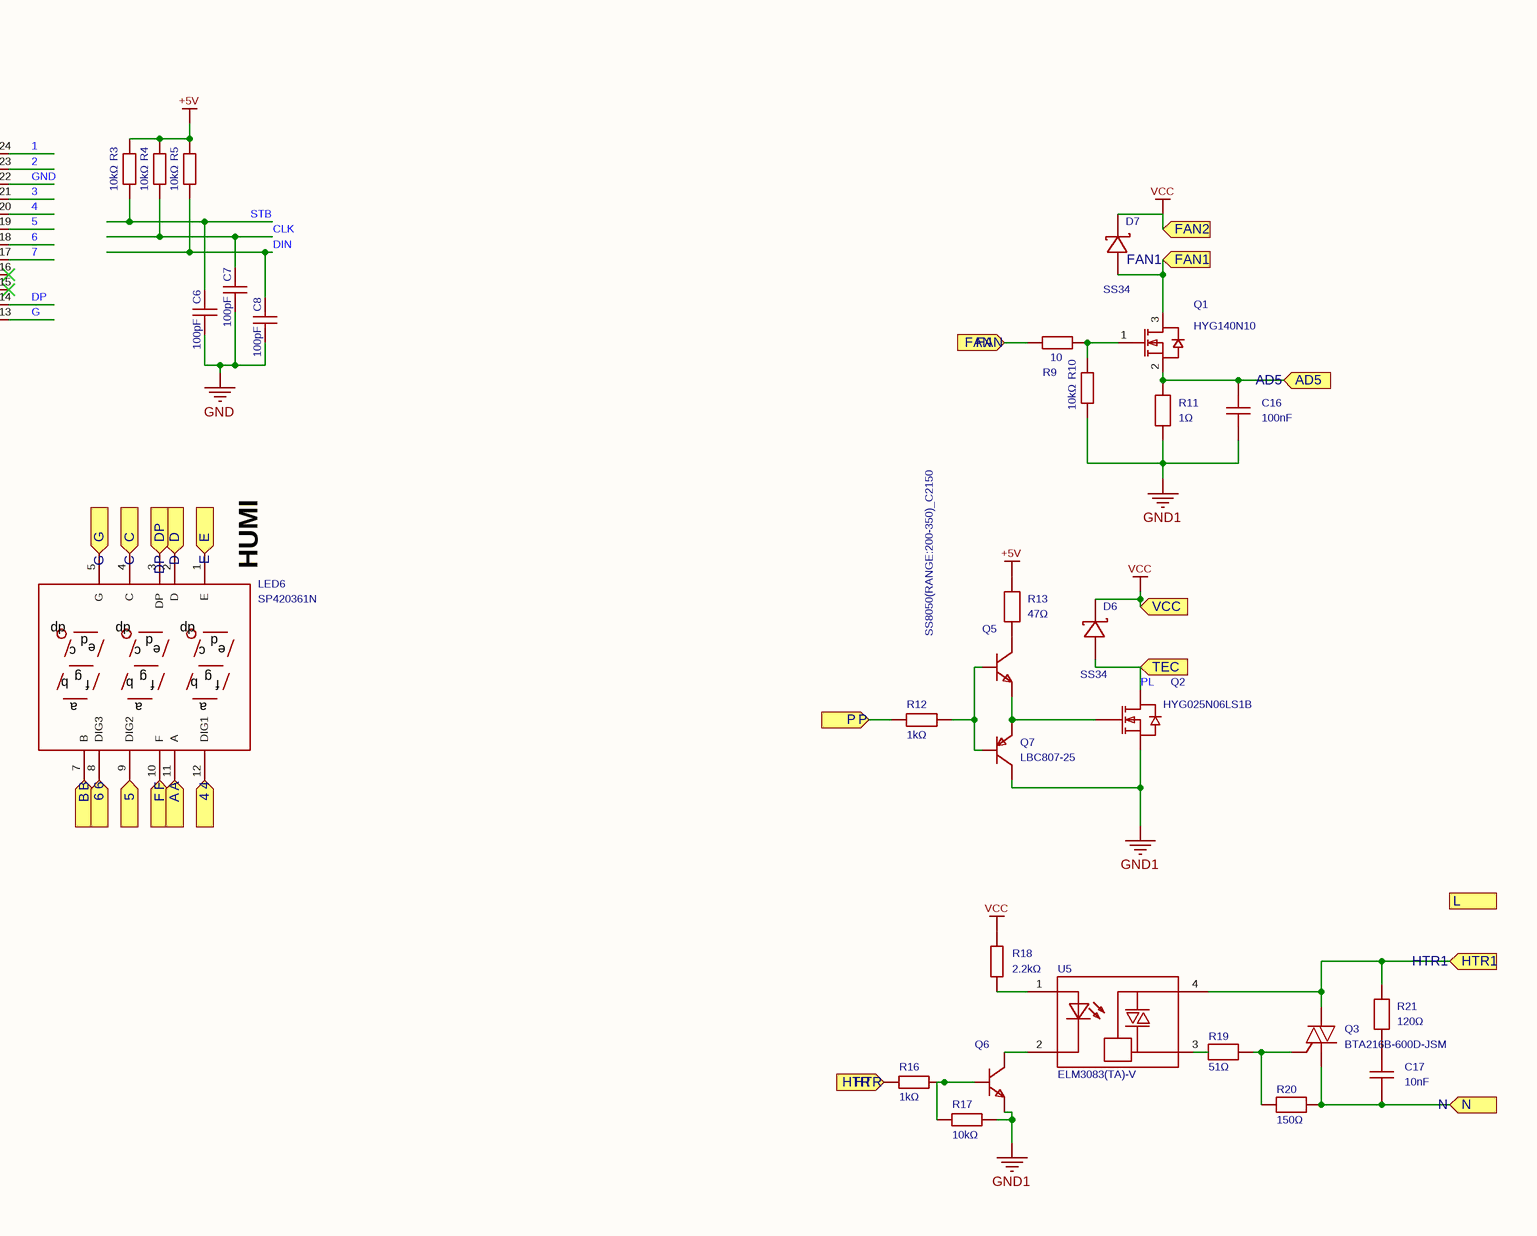
[diagram p0: MISC84275-2.SchDoc, right]
# Altium project MISC84275.PrjPcb (part 2 of 2)
## Sheet MISC84275-2.SchDoc (continued)
### Library data of the parts (continued)
D2 = SS34_C8678: Diode configuration:Single;Forward voltage(Vf):550mV@3A;DC reverse voltage(Vr):40V;Rectified current:3A;; Manufacturer: MDD(辰达半导体); AddInBom: yes; ModelId: e3551acb3c5a4975a5e9d36087fe1fa2; ModelTransform: 185.039,102.362,0,0,0,0,0,0,0; Diode Configuration: Single; Voltage - DC Reverse(Vr): 40V; Current - Rectified: 3A; Reverse Leakage Current (Ir): 500uA@40V; Operating Junction Temperature Range: -55℃~+125℃; Symbol: SS34_C8678; Device: SS34_C8678; LCSC Part Name: 电压:40V 电流:3A; SupplierPart: C8678; ManufacturerPart: SS34; Supplier Footprint: SMA(DO-214AC); JLCPCB Part Class: Basic library; Datasheet: https://item.szlcsc.com/datasheet/SS34/9178.html; Supplier: LCSC; ConvertToPcb: yes; FootprintName: SMA_L4.3-W2.6-LS5.2-RD; ModelName: SMA_L4.3-W2.6-LS5.2-RD; Voltage - Forward(Vf@If): 550mV@3A
D3-D5 = SMF36CA_C435502: Polarity:Bidirectional;Reverse standoff voltage(Vrwm):36V;Clamping voltage:58.1V;Peak pulse current(Ipp):3.5A;Peak pulse power(Ppp):200W@10/1000us;Breakdown voltage:40V;; Manufacturer: AnBon(安邦); 3D Model: 8576f175c34f41329e79954aa68cc529; 3D Model Transform: 145.669,70.866,0,0,0,0,0,0,0; Reverse Stand-Off Voltage (Vrwm): 36V; Clamping Voltage: 58.1V; Peak Pulse Current (Ipp): 3.5A; Voltage - Breakdown: 40V; Reverse Leakage Current (Ir): 5uA; Number of Channels: Single channel; Type: TVS; AddInBom: yes; Symbol: SMF36CA_C435502; Device: SMF36CA_C435502; LCSC Part Name: SMF36CA; Supplier Part: C435502; Manufacturer Part: SMF36CA; Supplier Footprint: SOD-123; JLCPCB Part Class: Extended library; Datasheet: https://item.szlcsc.com/datasheet/SMF36CA/432840.html; Supplier: LCSC; Polarity: Bidirectional; Peak Pulse Power Dissipation (Ppp): 200W@10/1000us; Operating Temperature: -55℃~+150℃; ConvertToPcb: yes; FootprintName: SOD-123_L2.7-W1.8-LS3.7-BI; ModelName: SOD-123_L2.7-W1.8-LS3.7-BI
D6 D7 = SS34_C8678: Diode configuration:Single;Forward voltage(Vf):550mV@3A;DC reverse voltage(Vr):40V;Rectified current:3A;; Manufacturer: MDD(辰达半导体); 3D Model: e3551acb3c5a4975a5e9d36087fe1fa2; 3D Model Transform: 185.039,102.362,0,0,0,0,0,0,0; Diode Configuration: Single; Voltage - DC Reverse(Vr): 40V; Current - Rectified: 3A; Reverse Leakage Current (Ir): 500uA@40V; Operating Junction Temperature Range: -55℃~+125℃; AddInBom: yes; Symbol: SS34_C8678; Device: SS34_C8678; LCSC Part Name: 电压:40V 电流:3A; Supplier Part: C8678; Manufacturer Part: SS34; Supplier Footprint: SMA(DO-214AC); JLCPCB Part Class: Basic library; Datasheet: https://item.szlcsc.com/datasheet/SS34/9178.html; Supplier: LCSC; Voltage - Forward(Vf@If): 550mV@3A; ConvertToPcb: yes; FootprintName: SMA_L4.3-W2.6-LS5.2-RD; ModelName: SMA_L4.3-W2.6-LS5.2-RD
FAN FAN2 = XH2.54-2P立贴: AddInBom: yes; ModelId: fc9104ee8bac4316b59c074360305c900819f05c4eef4c71ace90d822a990e87; ModelTransform: 393.7,326.771,0,0,0,0,0,9.966,0; Symbol: XH2.54-2P vertical SMD; Device: XH2.54-2P vertical SMD; LCSC Part Name: XH2.54-2P立贴; SupplierPart: C9900007402; ManufacturerPart: XH2.54-2P立贴; Supplier Footprint: XH2.5-2P母座立贴; JLCPCB Part Class: Extended Part; Supplier: LCSC; ConvertToPcb: yes; FootprintName: CONN-SMD_2P_A2501WV-S; ModelName: CONN-SMD_2P_A2501WV-S
H1 = PZ254V-11-04P: Pin structure:1x4P;Pitch:2.54mm;Row spacing:-;Round/square pin:Square pin;Mounting:Through-hole;Rows:Single row;Total pins:4P;Rated current:3A;Rated voltage:250V;Mating pin length:6mm;Body height:2.5mm;Tail length:3mm;Contact material:-;Operating temp:-40℃~+105℃;Colour:Black;; Manufacturer: XFCN(兴飞); Symbol: PZ254V-11-04P_C2691448; AddInBom: yes; ModelId: 112f4d05e8d64e99ab9a333894bea4f9; ModelName: HDR-TH_4P-P2.54-M-LI-1X4P; ModelTransform: 399.999,104.7242,0,0,0,0,0,0,-118.11; Pin Structure: 1x4P; Pitch: 2.54mm; Current Rating: 3A; Voltage Rating (Max): 250V; Device: PZ254V-11-04P; LCSC Part Name: 1x4P 间距:2.54mm 方针 直插; SupplierPart: C2691448; ManufacturerPart: PZ254V-11-04P; Supplier Footprint: 插件,P=2.54mm; JLCPCB Part Class: Extended library; Datasheet: https://item.szlcsc.com/datasheet/PZ254V-11-04P/2801085.html; Supplier: LCSC; ConvertToPcb: yes; FootprintName: HDR-TH_4P-P2.54-V-M; Row Spacing: -; Circluar Pins/Square Pins: Square pin; Mounting Type: Through-hole; Number of Rows: Single row; Number of Pins: 4P; Length of Mating Pin: 6mm; Insulation Height: 2.5mm; Length of End Connection Pin: 3mm; Contact Material: -; Operating Temperature: -40℃~+105℃; Color: Black
HTR = VH3.96-3P: AddInBom: yes; ModelId: 84617fe1842943989a766f28ebeae3030819f05c4eef4c71ace90d822a990e87; ModelTransform: 623.6208,484.251,0,0,0,0,0.001,0.984,0; Symbol: VH3.96-3P; Device: VH3.96-3P; LCSC Part Name: VH3.96-3P; SupplierPart: C9900014650; ManufacturerPart: VH3.96-3P; Supplier Footprint: VH3.963P贴; JLCPCB Part Class: Extended Part; Supplier: LCSC; ConvertToPcb: yes; FootprintName: CONN-SMD_3P-P3.96_HCTL_HC-VH-3ALT; ModelName: CONN-SMD_3P-P3.96_HCTL_HC-VH-3ALT
L1 = PSPMAA0605H-680M-IGF: Inductance:68uH;Tolerance:±20%;Rated current:1.5A;Saturation current(Isat):2A;Type:-;; Manufacturer: PROD(谱罗德); 3D Model: 42305e89796f47b49312a685ea93d4940819f05c4eef4c71ace90d822a990e87; 3D Model Transform: 275.59,259.88137,0,0,0,0,0,-0.551,0; Tolerance: ±20%; Current Rating: 1.5A; Current - Saturation(Isat): 2A; DC Resistance(DCR): 256mΩ; AddInBom: yes; ModelName: IND-SMD_L7.1-W6.6-H5.0; Symbol: PSPMAA0605H-680M-IGF; Device: PSPMAA0605H-680M-IGF; LCSC Part Name: 68uH ±20% 2A; Supplier Part: C2983094; Manufacturer Part: PSPMAA0605H-680M-IGF; Supplier Footprint: SMD,7.1x6.6mm; JLCPCB Part Class: Extended Part; Datasheet: https://item.szlcsc.com/datasheet/PSPMAA0605H-680M-IGF/3416346.html; Supplier: LCSC; Value: 68uH; Type: -; Ratings: -; ConvertToPcb: yes; FootprintName: IND-SMD_L7.1-W6.6_H5.0
L2 L3 = SCL3216T220KSP: Inductance:22uH;Tolerance:±10%;Rated current:5mA;Saturation current(Isat):-;DC resistance(DCR):900mΩ;; Manufacturer: Sunltech(顺磁); 3D Model: 85bdab7b3d4c4074b81d208eb5e865b30819f05c4eef4c71ace90d822a990e87; 3D Model Transform: 125.984,62.835,0,0,0,0,0,0,0; Tolerance: ±10%; Current Rating: 5mA; DC Resistance(DCR): 900mΩ; AddInBom: yes; ModelName: L1206_L3.2-W1.6-H1.1; Symbol: SCL3216T220KSP; Device: SCL3216T220KSP; LCSC Part Name: 22uH ±10%; Supplier Part: C412019; Manufacturer Part: SCL3216T220KSP; Supplier Footprint: 1206; JLCPCB Part Class: Extended Part; Datasheet: https://item.szlcsc.com/datasheet/SCL3216T220KSP/403512.html; Supplier: LCSC; Value: 22uH; Current - Saturation (Isat): -; Q @ Frequency: -; Frequency - Self Resonant: -; Ratings: -; ConvertToPcb: yes; FootprintName: L1206
LED1-LED4 = 3mmFIR: 3D Model: a497c992633541038a38947cdc58012f; 3D Model Transform: 141.274,153.327,0,0,0,0,-5.984,0,-137.795; AddInBom: yes; ModelName: LED-TH-3mm_R; Symbol: 3MMFIR; Device: 3mmFIR; LCSC Part Name: 3mmFIR; Supplier Part: C9900095018; Manufacturer Part: 3mmFIR; Supplier Footprint: LED-TH_LED-3MM_RED; JLCPCB Part Class: Extended library; Supplier: LCSC; ConvertToPcb: yes; FootprintName: LED-TH_BD3.0-P2.54-FD
LED5 LED6 = EPHB_SP420361N 0.36英寸3位红色数码管: Same display size as the 30V tester I bought, Digits:3 digits;Emitting colour:Red;LED polarity:Common cathode;Character height (inch):0.36;; Manufacturer: ARKLED(方舟); Device: EPHB_SP420361N 0.36 inch 3 digit red seven-segment display; 3D Model: 75b7188ef1934ceeb211c7922abf127e; 3D Model Transform: 885.825,551.5737,0,90,0,0,0,0,-196.85; Luminous Color: Red; Digit/Alpha Size(inch): 0.36; AddInBom: yes; Symbol: SP420361N; Manufacturer Part: SP420361N; Supplier: LCSC; Supplier Part: C98927; LCSC Part Name: 3位0.36英寸红色数码管 共阴极; Supplier Footprint: 插件; JLCPCB Part Class: Extended Part; Datasheet: https://atta.szlcsc.com/upload/public/pdf/source/20170713/C98927_1499918920582816853.pdf; Number of Characters: 3 digits; LED Polarity: Common cathode; ConvertToPcb: yes; FootprintName: LED-SEG-TH_SP420361N; ModelName: LED-SEG-TH_SP420361N
Q1 = NCE0140K2-VB: Type:1 N-channel;Drain-source voltage(Vdss):100V;Continuous drain current(Id):45A;On-resistance(RDS(on)@Vgs,Id):-;Power(Pd):3W;Threshold voltage(Vgs(th)@Id):2.5V@250uA;; Manufacturer: VBsemi(微碧半导体); 3D Model: 002f14490d3e47dc80a93c97f5a1e7bb; 3D Model Transform: 385.5088,255.905,0,0,0,0,-33.661,0,0; Drain Source Voltage (Vdss): 100V; Continuous Drain Current (Id): 45A; Power Dissipation (Pd): 3W; Total Gate Charge (Qg@Vgs): 38nC@10V; Input Capacitance (Ciss@Vds): 2.4nF@50V; Reverse Transfer Capacitance (Crss@Vds): 80pF@50V; AddInBom: yes; Symbol: NCE0140K2-VB; Device: NCE0140K2-VB; Manufacturer Part: HYG140N10; LCSC Part Name: 1个N沟道 耐压:100V 电流:45A; Supplier Part: C7463473; Supplier Footprint: TO-252; JLCPCB Part Class: Extended library; Datasheet: https://atta.szlcsc.com/upload/public/pdf/source/20240821/DCE0DDCDA6E2F6C426FEF52E9193F584.pdf; Supplier: LCSC; Type: 1 N-channel; Drain Source On Resistance (RDS(on)@Vgs,Id): -; Gate Threshold Voltage (Vgs(th)@Id): 2.5V@250uA; Operating Temperature: -55℃~+175℃; ConvertToPcb: yes; FootprintName: TO-252-3_L6.6-W6.1-P4.58-LS10.1-BR; ModelName: TO-252-3_L6.6-W6.1-P4.58-LS10.1-BR
Q2 = HYG025N06LS1B: Quantity:1 N-channel;Drain-source voltage(Vdss):60V;Continuous drain current(Id):160A;On-resistance(RDS(on)):3.3mΩ@10V;Power dissipation(Pd):125W;Threshold voltage(Vgs(th)):3V@250uA;; Manufacturer: HUAYI(华羿微); 3D Model: e74d9d1f92e14ef38b829eb45550a5f50819f05c4eef4c71ace90d822a990e87; 3D Model Transform: 399.999,594.487,0,90,0,0,-25.236,0,0; Drain to Source Voltage: 60V; Current - Continuous Drain(Id): 160A; Pd - Power Dissipation: 125W; Gate Charge(Qg): 58.3nC@10V; Input Capacitance(Ciss): 3.915nF; Reverse Transfer Capacitance (Crss@Vds): 10.2pF; Output Capacitance(Coss): 1.31nF; AddInBom: yes; Symbol: HYG025N06LS1B; Device: HYG025N06LS1B; LCSC Part Name: 1个N沟道 耐压:60V 电流:160A; Supplier Part: C2836680; Manufacturer Part: HYG025N06LS1B; Supplier Footprint: TO-263-2L; JLCPCB Part Class: Extended Part; Datasheet: https://item.szlcsc.com/datasheet/HYG025N06LS1B/3004274.html; Supplier: LCSC; Number: 1 N-channel; RDS(on): 3.3mΩ@10V; Gate Threshold Voltage (Vgs(th)): 3V@250uA; Operating Temperature: -55℃~+175℃; Type: N-channel; ConvertToPcb: yes; FootprintName: TO-263-2_L10.2-W8.7-P5.08-LS15.1-BR; ModelName: TO-263-2_L10.2-W8.7-P5.08-LS15.1-BR
Q3 = BTA216B-600D-JSM: Holding current(Ih):25mA;Off-state peak voltage(Vdrm):600V;Gate trigger current(Igt):50mA;; Manufacturer: JSMSEMI(杰盛微); 3D Model: 74c353bcc44b4c868478fa9e8b3e61680819f05c4eef4c71ace90d822a990e87; 3D Model Transform: 393.7,606.298,0,90,0,0,-49.213,0,0; Gate Trigger   Voltage (Vgt): 1.3V; Holding Current (Ih): 25mA; Peak off - state voltage(Vdrm): 600V; Current - Gate Trigger(Igt): 50mA; Voltage - On State(Vtm): 1.55V; Current - On State(It(RMS)): 16A; AddInBom: yes; Symbol: BTA216B-600D-JSM; Device: BTA216B-600D-JSM; LCSC Part Name: 16A无缓冲器三端双向可控硅; Supplier Part: C18189168; Manufacturer Part: BTA216B-600D-JSM; Supplier Footprint: TO-263; JLCPCB Part Class: Extended Part; Datasheet: https://item.szlcsc.com/datasheet/BTA216B-600D-JSM/19338246.html; Supplier: LCSC; ConvertToPcb: yes; FootprintName: TO-263-3_L10.2-W9.2-P5.08-LS15.4-BR; ModelName: TO-263-3_L10.2-W9.2-P5.08-LS15.4-BR
Q4-Q6 = SS8050(RANGE:200-350)_C2150: Transistor type:NPN;Collector current(Ic):1.5A;C-E breakdown voltage(Vceo):25V;Power(Pd):300mW;DC current gain(hFE@Ic,Vce):200@800mA,1V;; Manufacturer: CJ(江苏长电/长晶); Symbol: SS8050_C2150; 3D Model: c62791f0466c4ae2a892c056b845b0ca; 3D Model Transform: 98.425,114.173,0,180,0,0,0.0005,-0.0005,0; Transistor Type: NPN; Collector Current (Ic): 1.5A; Collector-Emitter Breakdown Voltage (Vceo): 25V; Power Dissipation (Pd): 300mW; Transition Frequency (fT): 100MHz; Collector Cut-Off Current (Icbo): 100nA; Collector-Emitter Saturation Voltage (VCE(sat)@Ic,Ib): 500mV@800mA,80mA; AddInBom: yes; ModelName: SOT-23-3P_L2.9-W1.3-H1.0-LS2.4-P0.95; Device: SS8050(RANGE:200-350)_C2150; LCSC Part Name: NPN 电流:1.5A 耐压:25V hfe=200~350; Supplier Part: C2150; Manufacturer Part: SS8050(RANGE:200-350); Supplier Footprint: SOT-23; JLCPCB Part Class: Basic library; Datasheet: https://atta.szlcsc.com/upload/public/pdf/source/20230322/AEE86F4B043774EFF80CAEA14A37D9E9.pdf; Supplier: LCSC; DC Current Gain (hFE@Ic,Vce): 200@800mA,1V; Operating Temperature: -55℃~+150℃; ConvertToPcb: yes; FootprintName: SOT-23-3_L2.9-W1.3-P1.90-LS2.4-BR
Q7 = LBC807-25LT1G: Transistor type:PNP;Collector current(Ic):500mA;C-E breakdown voltage(Vceo):45V;Power(Pd):225mW;DC current gain(hFE@Ic,Vce):160@100mA,1.0V;; Manufacturer: LRC(乐山无线电); 3D Model: 89cb27a44ab2466697082bb9fd73a7d0; 3D Model Transform: 114.173,110.236,0,90,0,0,0,0,0; Transistor Type: PNP; Collector Current (Ic): 500mA; Collector-Emitter Breakdown Voltage (Vceo): 45V; Power Dissipation (Pd): 225mW; Transition Frequency (fT): 100MHz; Collector Cut-Off Current (Icbo): 5uA; Collector-Emitter Saturation Voltage (VCE(sat)@Ic,Ib): 700mV@500mA,50mA; AddInBom: yes; ModelName: SOT-23-3L_L2.9-W1.6-H1.1-LS2.8-P0.95; Symbol: LBC807-25LT1G; Device: LBC807-25LT1G; Manufacturer Part: LBC807-25; LCSC Part Name: PNP 电流:500mA 耐压:45V hfe=160~400; Supplier Part: C12781; Supplier Footprint: SOT-23; JLCPCB Part Class: Extended library; Datasheet: https://atta.szlcsc.com/upload/public/pdf/source/20190627/C383184_22DCACC56563C88F03CAC9F09322D9FA.pdf; Supplier: LCSC; DC Current Gain (hFE@Ic,Vce): 160@100mA,1.0V; Operating Temperature: -55℃~+150℃; ConvertToPcb: yes; FootprintName: SOT-23-3_L2.9-W1.6-P1.90-LS2.8-BR
R1 R2 R12 R16 R23 = 0805W8F1001T5E: Resistor type:Thick film resistor;Resistance:1kΩ;Tolerance:±1%;Power:125mW;Max operating voltage:150V;Temp coefficient:±100ppm/℃;; Manufacturer: UNI-ROYAL(厚声); 3D Model: 37a81e68749a4138bd2dfa6897b24b850819f05c4eef4c71ace90d822a990e87; 3D Model Transform: 78.74,51.181,0,0,0,0,0,-0.0005,0; Tolerance: ±1%; Power(Watts): 125mW; Overload Voltage (Max): 150V; AddInBom: yes; ModelName: R0805_L2.0-W1.3-H0.6; Symbol: 0805W8F1001T5E; Device: 0805W8F1001T5E; LCSC Part Name: 1kΩ ±1% 125mW 厚膜电阻; Manufacturer Part: 0805W8F1001T5E; Supplier Footprint: 0805; JLCPCB Part Class: Basic Part; Datasheet: https://atta.szlcsc.com/upload/public/pdf/source/20200306/C422600_1E6D84923E4A46A82E41ADD87F860B5C.pdf; Supplier: LCSC; Type: Thick film resistor; Temperature Coefficient: ±100ppm/℃; Operating Temperature Range: -55℃~+155℃; ConvertToPcb: yes; FootprintName: R0805
  R1: Value: 1K
  R2: Value: 10kΩ
  R12 R16 R23: Supplier Part: C17513; Value: 1kΩ
R3-R5 R10 R17 R22 = 0805W8F1002T5E_C17414: Resistor type:Thick film resistor;Resistance:10kΩ;Tolerance:±1%;Power:125mW;Operating voltage:150V;Temp coefficient:±100ppm/℃;; Manufacturer: UNI-ROYAL(厚声); 3D Model: 37a81e68749a4138bd2dfa6897b24b850819f05c4eef4c71ace90d822a990e87; 3D Model Transform: 78.74,51.181,0,0,0,0,0,-0.0005,0; Tolerance: ±1%; Power(Watts): 125mW; Voltage-Supply(Max): 150V; AddInBom: yes; ModelName: R0805_L2.0-W1.3-H0.6; Symbol: 0805W8F1002T5E; Device: 0805W8F1002T5E_C17414; LCSC Part Name: 10kΩ ±1% 125mW 厚膜电阻; Supplier Part: C17414; Manufacturer Part: 0805W8F1002T5E; Supplier Footprint: 0805; JLCPCB Part Class: Basic Part; Datasheet: https://item.szlcsc.com/datasheet/0805W8F1002T5E/18102.html; Supplier: LCSC; Type: Thick film resistor; Value: 10kΩ; Temperature Coefficient: ±100ppm/℃; Operating Temperature: -55℃~+155℃; ConvertToPcb: yes; FootprintName: R0805
R6 R8 = 0805W8F4702T5E: Resistor type:Thick film resistor;Resistance:47kΩ;Tolerance:±1%;Power:125mW;Max operating voltage:150V;Temp coefficient:±100ppm/℃;; Manufacturer: UNI-ROYAL(厚声); 3D Model: 37a81e68749a4138bd2dfa6897b24b85; 3D Model Transform: 78.74,51.181,0,0,0,0,0,-0.0005,0; Tolerance: ±1%; Power(Watts): 125mW; Overload Voltage (Max): 150V; AddInBom: yes; ModelName: R0805_L2.0-W1.3-H0.6; Symbol: 0805W8F4702T5E; Device: 0805W8F4702T5E; LCSC Part Name: 47kΩ ±1% 125mW 厚膜电阻; Supplier Part: C17713; Manufacturer Part: 0805W8F4702T5E; Supplier Footprint: 0805; JLCPCB Part Class: Basic Part; Datasheet: https://atta.szlcsc.com/upload/public/pdf/source/20200306/C422600_1E6D84923E4A46A82E41ADD87F860B5C.pdf; Supplier: LCSC; Type: Thick film resistor; Value: 47kΩ; Temperature Coefficient: ±100ppm/℃; Operating Temperature Range: -55℃~+155℃; ConvertToPcb: yes; FootprintName: R0805
R7 = FRC0805F1202TS: Resistor type:Thick film resistor;Resistance:12kΩ;Tolerance:±1%;Power:125mW;Operating voltage:150V;Temp coefficient:±100ppm/℃;; Manufacturer: FOJAN(富捷); 3D Model: 37a81e68749a4138bd2dfa6897b24b850819f05c4eef4c71ace90d822a990e87; 3D Model Transform: 78.74,51.181,0,0,0,0,0,-0.0005,0; Tolerance: ±1%; Power(Watts): 125mW; Voltage-Supply(Max): 150V; AddInBom: yes; ModelName: R0805_L2.0-W1.3-H0.6; Symbol: FRC0805F1202TS; Device: FRC0805F1202TS; LCSC Part Name: 12kΩ ±1% 125mW 厚膜电阻; Supplier Part: C2907225; Manufacturer Part: FRC0805F1202TS; Supplier Footprint: 0805; JLCPCB Part Class: Extended Part; Supplier: LCSC; Type: Thick film resistor; Value: 12kΩ; Temperature Coefficient: ±100ppm/℃; Operating Temperature: -55℃~+155℃; ConvertToPcb: yes; FootprintName: R0805
R9 = Res_0805: Symbol: Resistor; 3D Model: 37a81e68749a4138bd2dfa6897b24b85; 3D Model Transform: 78.74,51.181,0,0,0,0,0,-0.0005,0; ConvertToPcb: yes; ModelName: R0805_L2.0-W1.3-H0.6; Device: Res_0805; Value: 10; Supplier Footprint: 0805; AddInBom: yes; FootprintName: R0805
R11 = FRC1206F1R00TS: Resistor type:Thick film resistor;Resistance:1Ω;Tolerance:±1%;Power:250mW;Operating voltage:200V;Temp coefficient:±200ppm/℃;; Manufacturer: FOJAN(富捷); AddInBom: yes; ModelId: 89a1f13db2384da588040e0b3c55bf660819f05c4eef4c71ace90d822a990e87; ModelName: R1206_L3.2-W1.6-H0.6; ModelTransform: 125.984,62.992,0,0,0,0,0,0,0; Tolerance: ±1%; Power(Watts): 250mW; Voltage-Supply(Max): 200V; Symbol: FRC1206F1R00TS; Device: FRC1206F1R00TS; LCSC Part Name: 1Ω ±1% 250mW 厚膜电阻; SupplierPart: C2907374; ManufacturerPart: FRC1206F1R00TS; Supplier Footprint: 1206; JLCPCB Part Class: Extended Part; Supplier: LCSC; ConvertToPcb: yes; FootprintName: R1206; Type: Thick film resistor; Value: 1Ω; Temperature Coefficient: ±200ppm/℃; Operating Temperature: -55℃~+155℃
R13 = TRC0805D47R0P0525Z: Resistance:47Ω;Tolerance:±0.5%;Temp coefficient:±25ppm/℃;; Manufacturer: EVER OHMS(天二科技); 3D Model: 37a81e68749a4138bd2dfa6897b24b85; 3D Model Transform: 78.74,51.181,0,0,0,0,0,-0.0005,0; Tolerance: ±0.5%; AddInBom: yes; ModelName: R0805_L2.0-W1.3-H0.6; Symbol: TRC0805D47R0P0525Z; Device: TRC0805D47R0P0525Z; LCSC Part Name: 47Ω ±0.5%; Supplier Part: C3202613; Manufacturer Part: TRC0805D47R0P0525Z; Supplier Footprint: 0805; Datasheet: https://atta.szlcsc.com/upload/public/pdf/source/20230427/2EEF059389940B3DFAA5C1B306F95C16.pdf; Supplier: LCSC; Value: 47Ω; Temperature Coefficient: ±25ppm/℃; Operating Temperature Range: -55℃~+155℃; ConvertToPcb: yes; FootprintName: R0805
R14 = Res_0603: Symbol: Resistor; 3D Model: fc143cca1e79419f9cd78b61e9279f08; 3D Model Transform: 31.8897,63.7794,0,90,0,0,0,0,0; ConvertToPcb: yes; Device: Res_0603; Supplier Footprint: 0603; Value: 0Ω; AddInBom: yes; FootprintName: R0603; ModelName: R0603
R18 = 0805W8F2201T5E: Resistor type:Thick film resistor;Resistance:2.2kΩ;Tolerance:±1%;Power:125mW;Operating voltage:150V;Temp coefficient:±100ppm/℃;; Manufacturer: UNI-ROYAL(厚声); AddInBom: yes; ModelId: 37a81e68749a4138bd2dfa6897b24b850819f05c4eef4c71ace90d822a990e87; ModelName: R0805_L2.0-W1.3-H0.6; ModelTransform: 78.74,51.181,0,0,0,0,0,-0.0005,0; Tolerance: ±1%; Power(Watts): 125mW; Voltage-Supply(Max): 150V; Symbol: 0805W8F2201T5E; Device: 0805W8F2201T5E; LCSC Part Name: 2.2kΩ ±1% 125mW 厚膜电阻; SupplierPart: C17520; ManufacturerPart: 0805W8F2201T5E; Supplier Footprint: 0805; JLCPCB Part Class: Basic Part; Datasheet: https://item.szlcsc.com/datasheet/0805W8F2201T5E/18208.html; Supplier: LCSC; ConvertToPcb: yes; FootprintName: R0805; Type: Thick film resistor; Value: 2.2kΩ; Temperature Coefficient: ±100ppm/℃; Operating Temperature: -55℃~+155℃
R19 = MMA02040C5109FB300: Resistor type:Thin film resistor;Resistance:51Ω;Tolerance:±1%;Power:400mW;Operating voltage:200V;Temp coefficient:±50ppm/℃;; Manufacturer: VISHAY(威世); 3D Model: bdd6039e5cb54d129162151e55f23c33; 3D Model Transform: 137.795,55.09383,0,0,0,0,0,0,0; Tolerance: ±1%; Power(Watts): 400mW; Voltage-Supply(Max): 200V; AddInBom: yes; Symbol: MMA02040C5109FB300; Device: MMA02040C5109FB300; LCSC Part Name: 薄膜电阻 51Ω ±1% 400mW; Supplier Part: C2078576; Manufacturer Part: MMA02040C5109FB300; Supplier Footprint: 0204; JLCPCB Part Class: Extended library; Datasheet: https://item.szlcsc.com/datasheet/MMA02040C5109FB300/2170163.html; Supplier: LCSC; Type: Thin film resistor; Value: 51Ω; Temperature Coefficient: ±50ppm/℃; Operating Temperature: -55℃~+155℃; ConvertToPcb: yes; FootprintName: R0204; ModelName: R0204
R20 = MMA02040E1500BB100: Resistor type:Thin film resistor;Resistance:150Ω;Tolerance:±0.1%;Power:250mW;Operating voltage:200V;Temp coefficient:±15ppm/℃;; Manufacturer: VISHAY(威世); 3D Model: bdd6039e5cb54d129162151e55f23c33; 3D Model Transform: 137.795,55.09383,0,0,0,0,0,0,0; Tolerance: ±0.1%; Power(Watts): 250mW; Voltage-Supply(Max): 200V; AddInBom: yes; Symbol: MMA02040E1500BB100; Device: MMA02040E1500BB100; LCSC Part Name: 薄膜电阻 150Ω ±0.1% 250mW; Supplier Part: C1848543; Manufacturer Part: MMA02040E1500BB100; Supplier Footprint: 0204; JLCPCB Part Class: Extended library; Datasheet: https://item.szlcsc.com/datasheet/MMA02040E1500BB100/1939356.html; Supplier: LCSC; Type: Thin film resistor; Value: 150Ω; Temperature Coefficient: ±15ppm/℃; Operating Temperature: -55℃~+125℃; ConvertToPcb: yes; FootprintName: R0204; ModelName: R0204
R21 = CSR0204FTDV1200: Resistance:120Ω;Tolerance:±1%;Power:250mW;Temp coefficient:±50ppm/℃;; Manufacturer: Viking(光颉); 3D Model: bdd6039e5cb54d129162151e55f23c33; 3D Model Transform: 137.795,55.09383,0,0,0,0,0,0,0; Tolerance: ±1%; Power(Watts): 250mW; AddInBom: yes; Symbol: CSR0204FTDV1200; Device: CSR0204FTDV1200; LCSC Part Name: 120Ω ±1% 250mW; Supplier Part: C724898; Manufacturer Part: CSR0204FTDV1200; Supplier Footprint: MELF-0204; JLCPCB Part Class: Extended library; Datasheet: https://item.szlcsc.com/datasheet/CSR0204FTDV1200/771603.html; Supplier: LCSC; Value: 120Ω; Temperature Coefficient: ±50ppm/℃; ConvertToPcb: yes; FootprintName: R0204; ModelName: R0204
SW1-SW4 = 1TS005F-2500-5001: Circuit:SPST;Button shape:Round button;Actuation force:2.5N;Mounting:Vertical SMD;Switch length:6mm;Switch width:6mm;Switch height:5mm;Bracket:Without bracket;Contact current:50mA;Rated voltage:12V;Lamp:None;Life:7 ten-thousand cycles;; Manufacturer: HYP(鸿源精密); Circuit: SPST; Operating Force: 2.5N; Switch Height: 5mm; Contact Current: 50mA; Voltage Rating: 12V; Actuator/Cap Color: Black; With Lamp: None; 3D Model: f7f45881e00548f6bcbc5adaea3b18e7; 3D Model Transform: 354.33,236.614,0,0,0,0,0,0,0; AddInBom: yes; Symbol: 1TS005F-2500-5001; Device: 1TS005F-2500-5001; LCSC Part Name: 6*6*5mm 立贴 轻触开关; Supplier Part: C255812; Manufacturer Part: 1TS005F-2500-5001; Supplier Footprint: SMD,6x6mm; JLCPCB Part Class: Extended library; Datasheet: https://atta.szlcsc.com/upload/public/pdf/source/20180720/C255812_0808C7D708FD1FB7246546D29134BBAD.pdf; Supplier: LCSC; Actuator Style: Round button; Mounting Type: Vertical SMD; Length: 6mm; Width: 6mm; with Bracket: Without bracket; Termination Style: Gull-wing; Life: 7 ten-thousand cycles; Operating Temperature: -40℃~+90℃; ConvertToPcb: yes; FootprintName: SW-SMD_4P-L6.0-W6.0-P4.50-LS9.0-H2.5; ModelName: SW-SMD_4P-L6.0-W6.0-P4.50-LS9.0-H2.5
U1 = LCM08F003: AddInBom: yes; ModelId: c491f68934b34c649df5890a1d97cd0f0819f05c4eef4c71ace90d822a990e87; ModelName: TSSOP-20_L6.5-W4.4-H1.0-LS6.4-P0.65; ModelTransform: 251.969,255.906,0,90,0,0,0.0005,0,0; Symbol: LCM08F003; Device: LCM08F003; Manufacturer Part: TSSOP-20; LCSC Part Name: LCM08F003; SupplierPart: C9900009866; Supplier Footprint: TSSOP-20; JLCPCB Part Class: Extended Part; Supplier: LCSC; ConvertToPcb: yes; FootprintName: TSSOP-20_L6.5-W4.4-P0.65-LS6.4-BL
U3 = XL1509-5.0: Function:Buck;Output type:Fixed;Operating voltage:4.5V~40V;Output voltage:5V;Output current:2A;; Manufacturer: UMW(友台半导体); Symbol: XL1509-5.0_C2902368; AddInBom: yes; ModelId: e81d2f7d937b4a6ab1dca543ff5d56a4; ModelName: SOIC-8_L4.9-W3.9-H1.7-LS6.0-P1.27; ModelTransform: 189.751,236.22,0,180,0,0,0,0,0; Function: Buck; Output Type: Fixed; Output Voltage: 5V; Output Current: 2A; Switching Frequency: 150kHz; Synchronous Rectification: No; Number of Outputs: 1; Quiescent Current (Iq): 150uA; Switch tube (built-in/external): Built-in; Device: XL1509-5.0; LCSC Part Name: 150 KHz 固定频率 PWM 降压 DC/DC 转换器; SupplierPart: C2902368; ManufacturerPart: XL1509-5.0; Supplier Footprint: SOIC-8; JLCPCB Part Class: Extended library; Datasheet: https://atta.szlcsc.com/upload/public/pdf/source/20241113/D9907419AB21EE12D855D7DFAFDDCB19.pdf; Supplier: LCSC; ConvertToPcb: yes; FootprintName: SOIC-8_L4.9-W3.9-P1.27-LS6.0-TR; Input Voltage: 4.5V~40V; Operating Temperature: -40℃~+125℃; Topology: Buck
U4 = MAX485ESA(UMW): Manufacturer: UMW(友台半导体); Symbol: MAX485EAS; 3D Model: a3315c1c78f949e6bb82c6eaca1c53c7; 3D Model Transform: 244.094,196.85,0,90,0,0,0,0,0; AddInBom: yes; ModelName: SOP-8_L5.0-W4.0-H1.8-LS6.2-P1.27; Device: MAX485ESA(UMW); LCSC Part Name: MAX485ESA; Supplier Part: C668206; Manufacturer Part: MAX485ESA(UMW); Supplier Footprint: SOP-8; JLCPCB Part Class: Extended library; Datasheet: https://atta.szlcsc.com/upload/public/pdf/source/20241113/10AF97024436AF2218887750501B1DE1.pdf; Supplier: LCSC; ConvertToPcb: yes; FootprintName: SOP-8_L5.0-W4.0-P1.27-LS6.0-BL
U5 = ELM3083(TA)-V: Forward voltage:1.5V;Forward current:60mA;Load voltage:800V;Static dv/dt:1000V/us;; Manufacturer: EVERLIGHT(亿光); 3D Model: 7a816c7b730e4b8989440f8e2ea085d3; 3D Model Transform: 157.48,275.591,0,270,0,0,0,0,0; Zero Crossing Circuit: Yes; Forward Voltage: 1.5V; Isolation Voltage(rms): 3.75kV; Forward Current: 60mA; Load Voltage: 800V; Number of Outputs: 1; ModelName: SOP-4_L4.0-W4.4-H2.1-LS7.0-P2.54; Symbol: ELM3083(TA)-V; Device: ELM3083(TA)-V; LCSC Part Name: 可控硅光耦; Supplier Part: C5200145; Manufacturer Part: ELM3083(TA)-V; Supplier Footprint: SOP-4-2.54mm; JLCPCB Part Class: Extended library; Datasheet: https://atta.szlcsc.com/upload/public/pdf/source/20221025/E6F9D0F1F8000162E7F62C18F1E632B6.pdf; Supplier: LCSC; Static dv/dt: 1000V/us; Operating Temperature: -40℃~+110℃; AddInBom: yes; ConvertToPcb: yes; FootprintName: SOP-4_L4.4-W4.0-P2.54-LS7.0-TL
U6 = TM1668-SSOP24-TA2108: Type:-;Operating voltage(DC):3V~6V;Switching frequency:-;Channels:-;Output voltage:-;Output current:-;Dimming:-;Topology:-;; Manufacturer: TM(天微); AddInBom: yes; ModelId: f5b2473ce40e4151ba004f11ac5dda6c0819f05c4eef4c71ace90d822a990e87; ModelName: SSOP-24_L8.2-W5.3-H1.8-LS7.8-P0.65; ModelTransform: 322.834,307.086,0,0,0,0,0,0,0; Voltage - Input(DC): 3V~6V; Symbol: TM1668-SSOP24-TA2108; Device: TM1668-SSOP24-TA2108; LCSC Part Name: LED驱动控制专用电路; SupplierPart: C42418156; ManufacturerPart: TM1668-SSOP24-TA2108; Supplier Footprint: SSOP-24; Datasheet: https://item.szlcsc.com/datasheet/TM1668-SSOP24-TA2108/44424498.html; Supplier: LCSC; ConvertToPcb: yes; FootprintName: SSOP-24_L8.1-W5.3-P0.65-LS7.8-BL; Type: -; Frequency - Switching: -; Number of Channels: -; Output Voltage: -; Output Current: -; Dimming: -; Features: -; Voltage - Input(AC): -; Topology: -; Operating temperature: -40℃~+85℃; Switch Tube (Built-In/External): -; Constant Current Accuracy: -